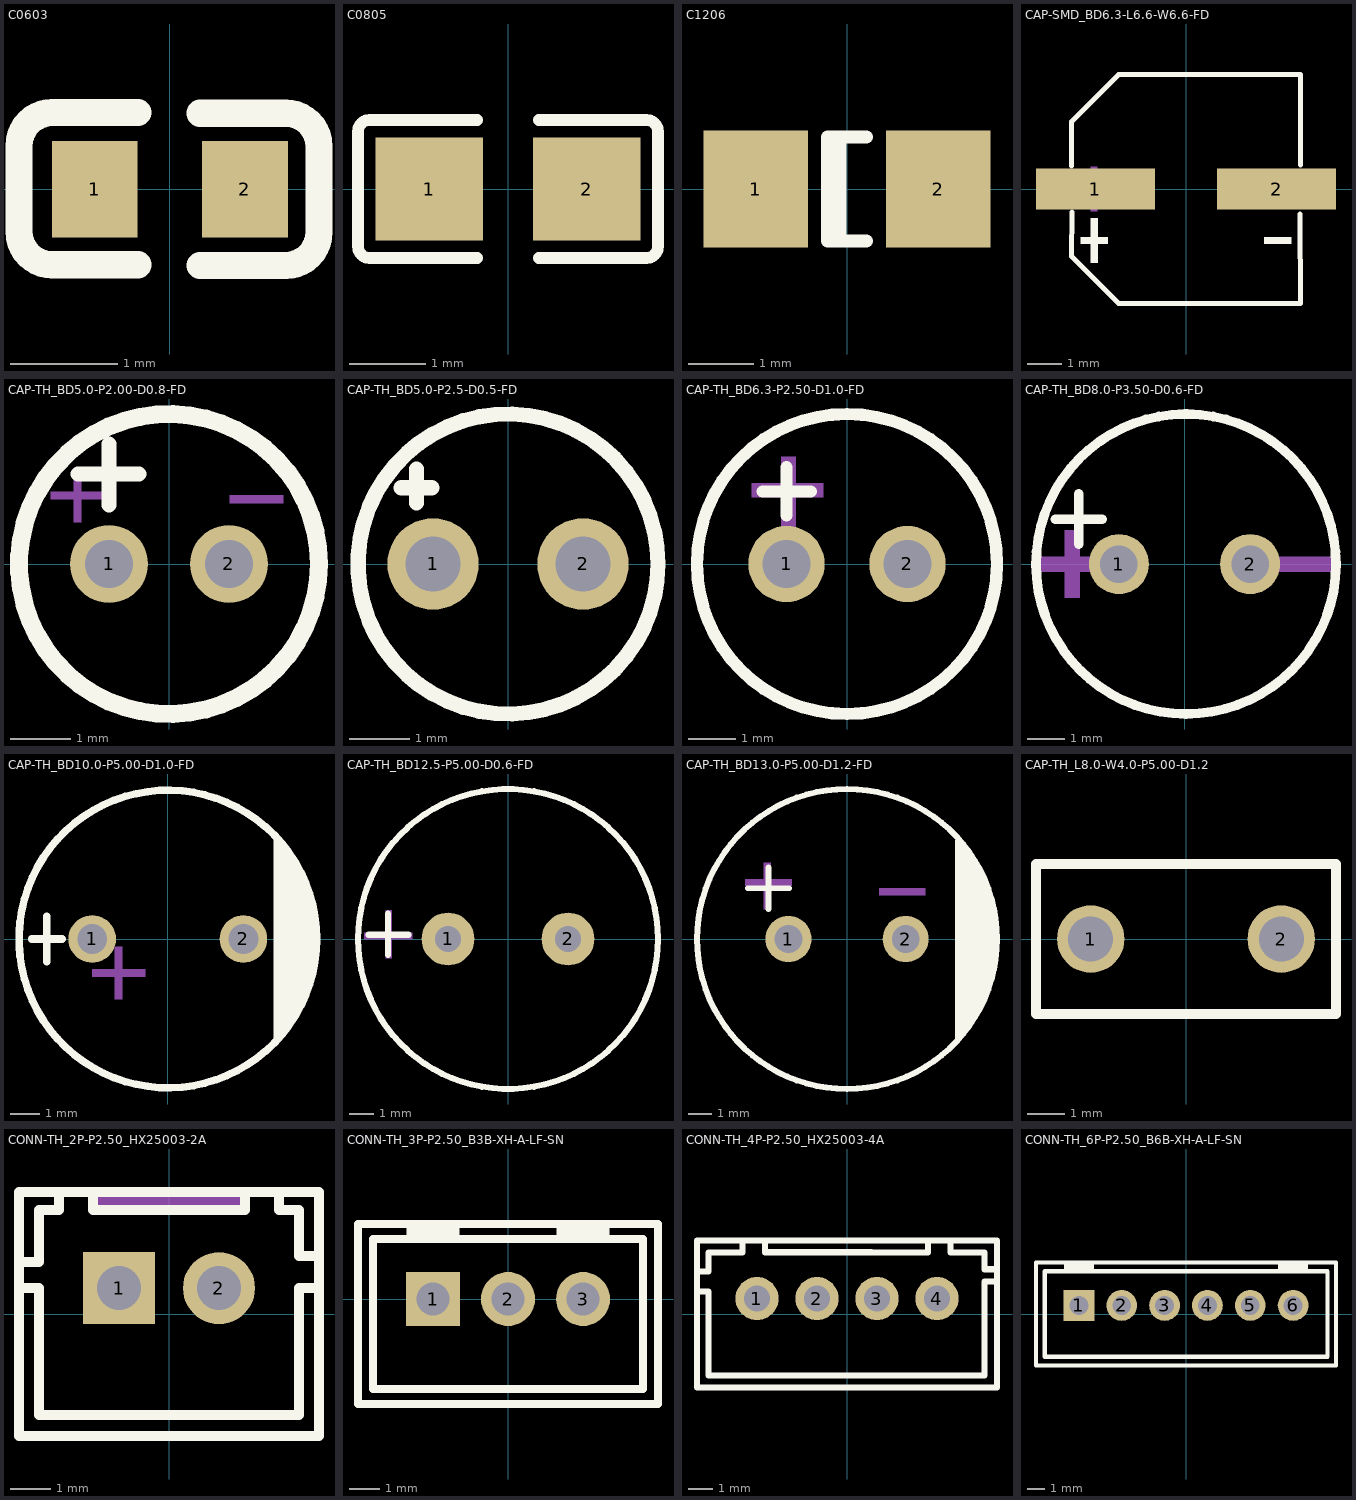
[diagram p0: the footprints below, top view; thin cyan lines are the x and y axes]
# Altium footprint library MISC84402-2.PcbLib: 69 footprints (part 1 of 5)
Each footprint in its own frame and in the unit in brackets; x right, y up, seen from the top. Pads: shape width x height; smd on the part's side, far side on the other; paste and mask are expansions set on the pad; w line width, h text height; cw(c..) or ccw(c..) is an arc to the next point about the centre after c.

## C0603 [mm]
height 12.5
pads (2):
  rect 0.8x0.9 smd: 1(-0.7,0) 2(0.7,0)
Top Overlay:
  lines w0.254: -0.296,-0.704 -1.096,-0.704 cw(c-1.096,-0.394) -1.406,-0.394 -1.405,0.406 cw(c-1.096,0.406) -1.096,0.715 -0.296,0.715 ; 0.28,-0.71 1.08,-0.71 ccw(c1.08,-0.4) 1.39,-0.4 1.39,0.4 ccw(c1.08,0.4) 1.08,0.71 0.28,0.71

## C0805 [mm]
pads (2):
  rect 1.41x1.35 smd: 1(-1.03,0) 2(1.03,0)
Top Overlay:
  lines w0.152: -0.401,-0.904 -1.811,-0.904 cw(c-1.811,-0.751) -1.964,-0.751 -1.964,0.751 cw(c-1.811,0.751) -1.811,0.904 -0.401,0.904 ; 0.401,-0.904 1.811,-0.904 ccw(c1.811,-0.751) 1.964,-0.751 1.964,0.751 ccw(c1.811,0.751) 1.811,0.904 0.401,0.904
Top Paste:
  region: 0.475,-0.62 0.475,-0.2 0.92,-0.2 0.92,0.25 0.48,0.25 0.475,0.66 0.525,0.71 1.675,0.71 1.725,0.66 1.725,-0.62 1.675,-0.67 0.525,-0.67
  region: -1.675,-0.62 -1.675,0.66 -1.625,0.71 -0.475,0.71 -0.425,0.66 -0.42,0.25 -0.87,0.25 -0.87,-0.2 -0.43,-0.2 -0.425,-0.62 -0.475,-0.67 -1.625,-0.67

## C1206 [mm] "Chip Capacitor; Body 3.2 x 1.6 mm (LxW typ)"
height 1.35
pads (2):
  rect 1.6x1.8 smd: 1(-1.4,0) 2(1.4,0)
Top Overlay:
  lines w0.2: -0.11,-0.8 -0.11,0.8 ; 0.3,-0.8 -0.3,-0.8 -0.3,0.8 0.3,0.8

## CAP-SMD_BD6.3-L6.6-W6.6-FD [mm]
pads (2):
  rect 3.5x1.2 smd: 1(-2.67,0) 2(2.67,0)
Top Overlay:
  region: 3.102,-1.419 3.102,-1.617 2.31,-1.617 2.31,-1.419
  region: -3.102,-1.419 -3.102,-1.617 -2.31,-1.617 -2.31,-1.419
  region: -2.805,-0.858 -2.805,-2.178 -2.607,-2.178 -2.607,-0.858
  lines w0.152: -3.376,0.686 -3.376,1.98 -1.98,3.376 3.376,3.376 3.369,0.707 ; -3.362,-0.686 -3.376,-1.981 -1.981,-3.376 3.376,-3.376 3.356,-0.74
Mechanical 15:
  region: 3.102,0.099 3.102,-0.099 2.31,-0.099 2.31,0.099
  region: -3.102,0.099 -3.102,-0.099 -2.31,-0.099 -2.31,0.099
  region: -2.81,0.66 -2.81,-0.66 -2.612,-0.66 -2.612,0.66

## CAP-TH_BD5.0-P2.00-D0.8-FD [mm]
pads (2):
  round 1.3 hole 0.8: 1(-1,0) 2(1,0)
Top Overlay:
  circle w0.3: c0,0 r2.5
  lines w0.254: -1.516,1.5 -0.5,1.5 ; -1,0.984 -1,2
Mechanical 15:
  region: -1.969,1.206 -1.08,1.206 -1.08,1.079 -1.969,1.079
  region: -1.588,0.699 -1.588,1.587 -1.461,1.587 -1.46,0.699
  region: 1.016,1.143 1.905,1.143 1.905,1.016 1.016,1.016

## CAP-TH_BD5.0-P2.5-D0.5-FD [mil]
pads (2):
  round 60 hole 36: 1(-49.21,0) 2(49.21,0)
Top Overlay:
  circle w10: c0,0 r98.43
  lines w10: -70,50 -50,50 ; -60,40 -60,62.4

## CAP-TH_BD6.3-P2.50-D1.0-FD [mm]
pads (2):
  round 1.6 hole 1: 1(-1.27,0) 2(1.27,0)
Top Overlay:
  circle w0.254: c0,0 r3.15
  lines w0.254: -1.778,1.524 -0.762,1.524 ; -1.27,1.016 -1.27,2.032
Mechanical 15:
  region: -2,1.7 -0.5,1.7 -0.5,1.4 -2,1.4
  region: -1.381,0.752 -1.381,2.252 -1.081,2.252 -1.081,0.752

## CAP-TH_BD8.0-P3.50-D0.6-FD [mm]
pads (2):
  round 1.6 hole 1: 1(-1.75,0) 2(1.75,0)
Top Overlay:
  lines w0.254: -3.445,1.2 -2.2,1.2 ; -2.822,0.527 -2.822,1.873 ; 0.003,4 ccw(c0.038,0.001) 0.074,4
Mechanical 15:
  region: -3.2,-0.9 -2.8,-0.9 -2.8,0.9 -3.2,0.9
  region: -3.9,0.2 -3.9,-0.2 -2.1,-0.2 -2.1,0.2
  region: 2.1,0.2 2.1,-0.2 3.9,-0.2 3.9,0.2

## CAP-TH_BD10.0-P5.00-D1.0-FD [mm]
pads (2):
  round 1.6 hole 1: 1(-2.54,0) 2(2.54,0)
Top Overlay:
  circle w0.254: c0,0 r5
  region: 3.556,3.556 3.556,-3.556 4.318,-2.54 4.826,-1.016 5.08,0.508 4.826,1.524
  lines w0.254: -4.572,0 -3.556,0 ; -4.064,-0.762 -4.064,0.762
Mechanical 15:
  region: -1.778,-2.032 -1.524,-2.032 -1.524,-0.254 -1.778,-0.254
  region: -2.54,-1.016 -0.762,-1.016 -0.762,-1.27 -2.54,-1.27

## CAP-TH_BD12.5-P5.00-D0.6-FD [mm]
pads (2):
  round 2.2 hole 1.1: 1(-2.5,0) 2(2.5,0)
Top Overlay:
  circle w0.254: c0,0 r6.25
  lines w0.254: -5.817,0.178 -4.14,0.178 ; -5.004,-0.66 -5.004,1.067
Mechanical 15:
  region: -6,0.25 -4,0.25 -4,0 -6,0
  region: -5.092,-0.811 -5.092,1.189 -4.842,1.189 -4.842,-0.811

## CAP-TH_BD13.0-P5.00-D1.2-FD [mm]
pads (2):
  round 2 hole 1.2: 1(-2.539,0) 2(2.541,0)
Top Overlay:
  circle w0.254: c0,0 r6.5
  region: 4.701,4.3 4.701,-4.5 5.801,-3 6.301,-1.7 6.401,-0.5 6.301,1.5 5.701,3.2
  lines w0.254: -4.3,2.2 -2.5,2.2 ; -3.4,1.3 -3.4,3.1
Mechanical 15:
  region: 4.722,4.286 4.722,-4.514 5.822,-3.014 6.322,-1.714 6.422,-0.514 6.322,1.486 5.722,3.186
  region: -4.399,2.6 -2.399,2.6 -2.399,2.3 -4.399,2.3
  region: -3.599,1.3 -3.599,3.3 -3.499,3.3 -3.299,3.3 -3.299,1.3
  region: 1.401,2.2 3.401,2.2 3.401,1.9 1.401,1.9

## CAP-TH_L8.0-W4.0-P5.00-D1.2 [mm]
pads (2):
  round 1.8 hole 1.2: 1(-2.54,0) 2(2.54,0)
Top Overlay:
  lines w0.254: -4,-2 4,-2 4,2 -4,2 -4,-2

## CONN-TH_2P-P2.50_HX25003-2A [mm]
pads (2):
  rect 1.8x1.8 hole 1.1: 1(-1.25,0.646)
  round 1.8 hole 1.1: 2(1.25,0.646)
Top Overlay:
  lines w0.254: -3.75,-1.769 -3.75,0.646 -3.25,0.646 -3.25,-1.769 -3.25,-2.521 3.25,-2.521 3.25,-1.698 3.25,0.646 3.75,0.646 3.75,-1.698 ; -3.75,-0.957 -3.75,1.294 -3.25,1.296 -3.25,2.604 -2.75,2.604 -2.75,3.054 ; -1.9,2.596 -1.9,3.046 ; -1.9,2.604 1.9,2.604 ; 1.9,2.596 1.9,3.046 ; 2.75,2.596 2.75,3.045 ; 2.75,2.604 3.25,2.604 3.25,1.446 3.75,1.446 3.75,-0.855 ; -3.75,-3.054 -3.75,3.046 3.75,3.046 3.75,-3.054 -3.75,-3.054
Mechanical 15:
  region: 1.9,3.046 1.9,2.546 -1.9,2.546 -1.9,3.046

## CONN-TH_3P-P2.50_B3B-XH-A-LF-SN [mm]
pads (3):
  rect 1.8x1.8 hole 1.1: 1(-2.5,0)
  round 1.8 hole 1.1: 2(0,0) 3(2.5,0)
Top Overlay:
  lines w0.254: -3.251,1.999 -3.251,2.499 ; -3.251,2.25 -1.749,2.25 ; -1.749,1.999 -1.749,2.499 ; 1.75,2.001 1.75,2.501 ; 1.75,2.251 3.25,2.251 ; 3.25,2.001 3.25,2.501 ; -5,-3.499 4.999,-3.499 4.999,2.5 -5,2.5 -5,-3.499 ; -4.5,-2.999 4.5,-2.999 4.5,2 -4.5,2 -4.5,-2.999

## CONN-TH_4P-P2.50_HX25003-4A [mm]
pads (4):
  round 1.8 hole 1.1: 1(-3.75,0.645) 2(-1.25,0.645) 3(1.25,0.645) 4(3.75,0.645)
Top Overlay:
  lines w0.254: -6.25,-3.055 -6.25,3.045 ; -6.25,-3.055 6.25,-3.055 ; -6.25,1.775 -5.775,1.775 -5.775,2.57 -4.361,2.57 -4.361,3.02 ; -6.25,3.055 6.24,3.055 ; -6.24,0.945 -5.775,0.945 -5.775,-2.555 5.726,-2.555 5.726,1.356 6.226,1.356 ; -3.424,3.021 -3.424,2.571 1.019,2.571 0.976,2.57 ; 1.019,2.57 3.375,2.57 3.375,3.02 ; 4.31,2.571 4.31,3.019 ; 4.314,2.57 5.726,2.57 5.726,1.864 6.226,1.864 ; 6.25,-3.055 6.25,3.045

## CONN-TH_6P-P2.50_B6B-XH-A-LF-SN [mm]
pads (6):
  rect 1.8x1.8 hole 1.1: 1(-6.251,0.501)
  round 1.8 hole 1.1: 2(-3.749,0.499) 3(-1.249,0.499) 4(1.251,0.499) 5(3.751,0.499) 6(6.251,0.499)
Top Overlay:
  lines w0.254: -7,2.5 -7,3 ; -7,2.75 -5.5,2.75 ; -5.5,2.5 -5.5,3 ; 5.501,2.5 5.501,3 ; 5.501,2.75 7.001,2.75 ; 7.001,2.5 7.001,3 ; -8.75,-3 8.75,-3 8.75,3 -8.75,3 -8.75,-3 ; -8.25,-2.5 8.251,-2.5 8.251,2.5 -8.25,2.5 -8.25,-2.5